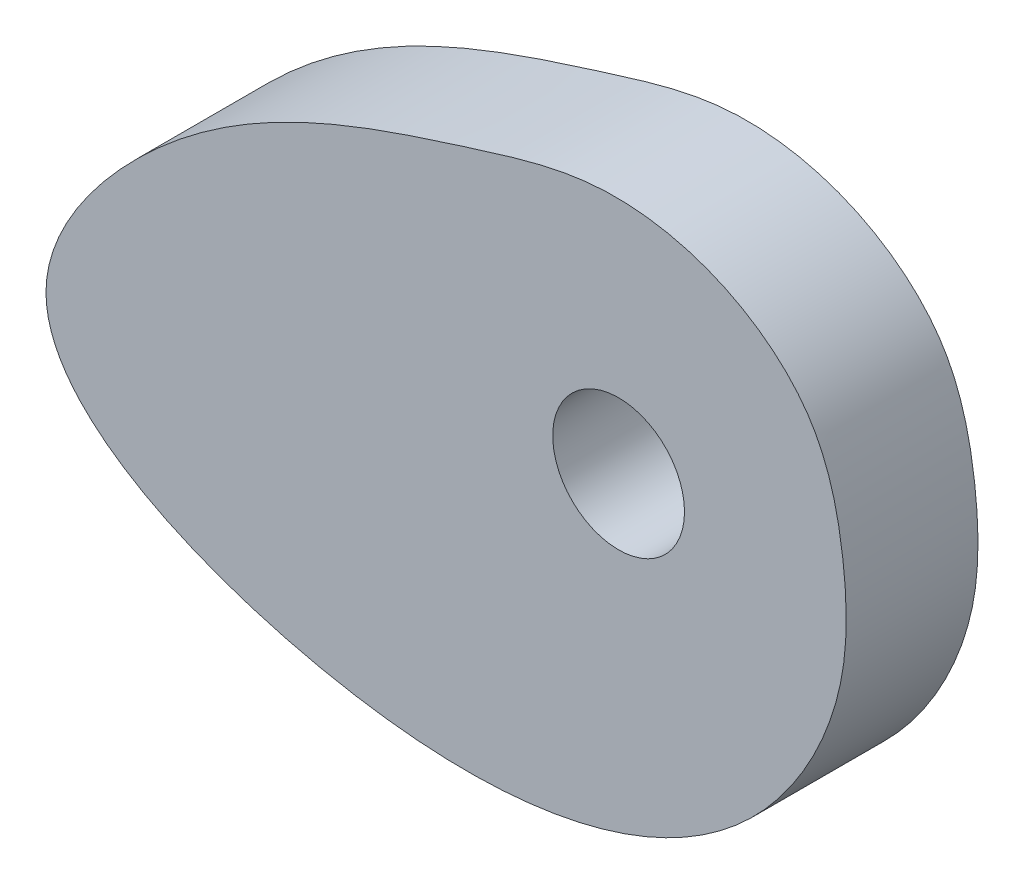
from build123d import *

# Parameters (mm, degrees)
SKETCH1_R           = 5
BOSS_EXTRUDE1_DEPTH = 10


with BuildPart() as part:
    # Sketch1 → Boss-Extrude1 (new body)
    with BuildSketch(Plane.XY):
        with BuildLine():
            add(Edge.make_bspline(
                [(17.012517442, 2.957517207), (16.670478453, 5.672178927), (15.376695719, 11.265953823), (7.999602539, 17.177874454), (-1.479494805, 18.808508667), (-16.414530478, 14.212952947), (-32.420198414, 9.013909894), (-50.269600748, -14.108282025), (-17.23472676, -28.814390043), (9.041241393, -23.634721545), (17.515245457, -6.090805118), (17.323703177, 0.487728599), (17.012517442, 2.957517207)],
                knots=[0, 0, 0, 0, 0.050620928, 0.103696373, 0.166927343, 0.223625645, 0.393033325, 0.496899233, 0.659127768, 0.876666263, 0.953945278, 1, 1, 1, 1], degree=3))
        make_face()
        Circle(SKETCH1_R, mode=Mode.SUBTRACT)
    extrude(amount=BOSS_EXTRUDE1_DEPTH)


solid = part.part
